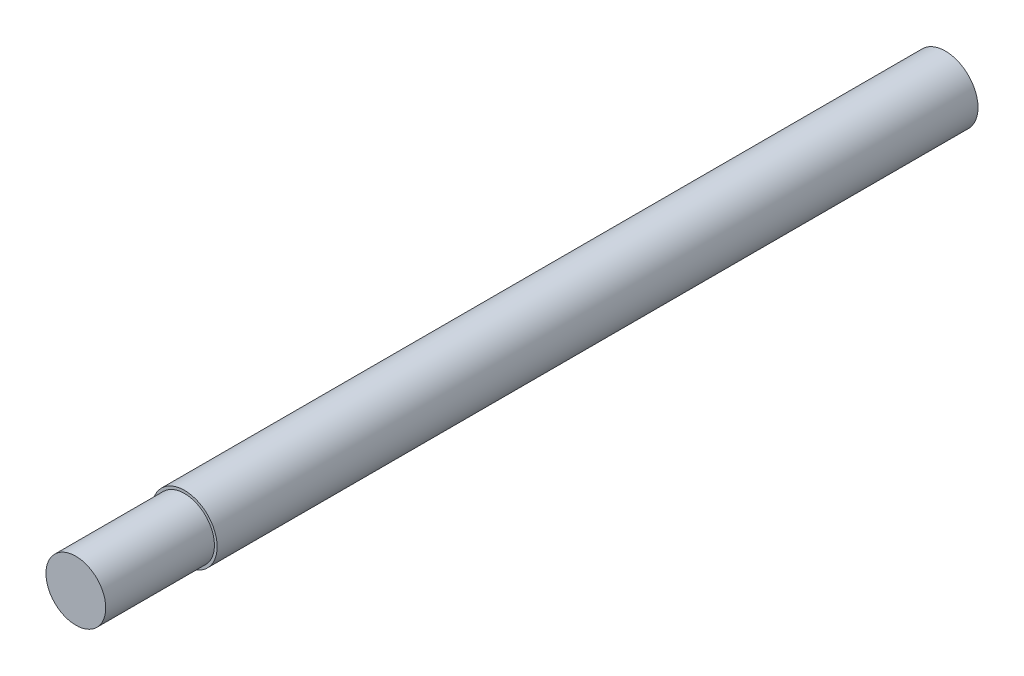
SolidWorks part; units mm, degrees
ref_plane "前视基准面" through (0, 0, 0) normal (0, 0, 1) x (1, 0, 0)
ref_plane "上视基准面" through (0, 0, 0) normal (0, 1, 0) x (1, 0, 0)
ref_plane "右视基准面" through (0, 0, 0) normal (1, 0, 0) x (0, 0, -1)
sketch "草图1" plane through (0, 0, 0) normal (0, 0, 1) x (1, 0, 0)
  circle A0 centre (0, 0) radius 6
  dimension "D1" = 12
extrude "凸台-拉伸3" add sketch "草图1" along normal mid plane 160
sketch "草图3" plane through (0, 0, 80) normal (0, 0, 1) x (1, 0, 0)
  circle A0 centre (0, 0) radius 5.5
  circle A1 centre (0, 0) radius 6 construction
  circle A2 centre (0, 0) radius 6
  dimension "D1" = 11
extrude "切除-拉伸1" cut sketch "草图3" against normal blind 20
cosmetic thread "装饰螺纹线1" parameters "D2"=10
